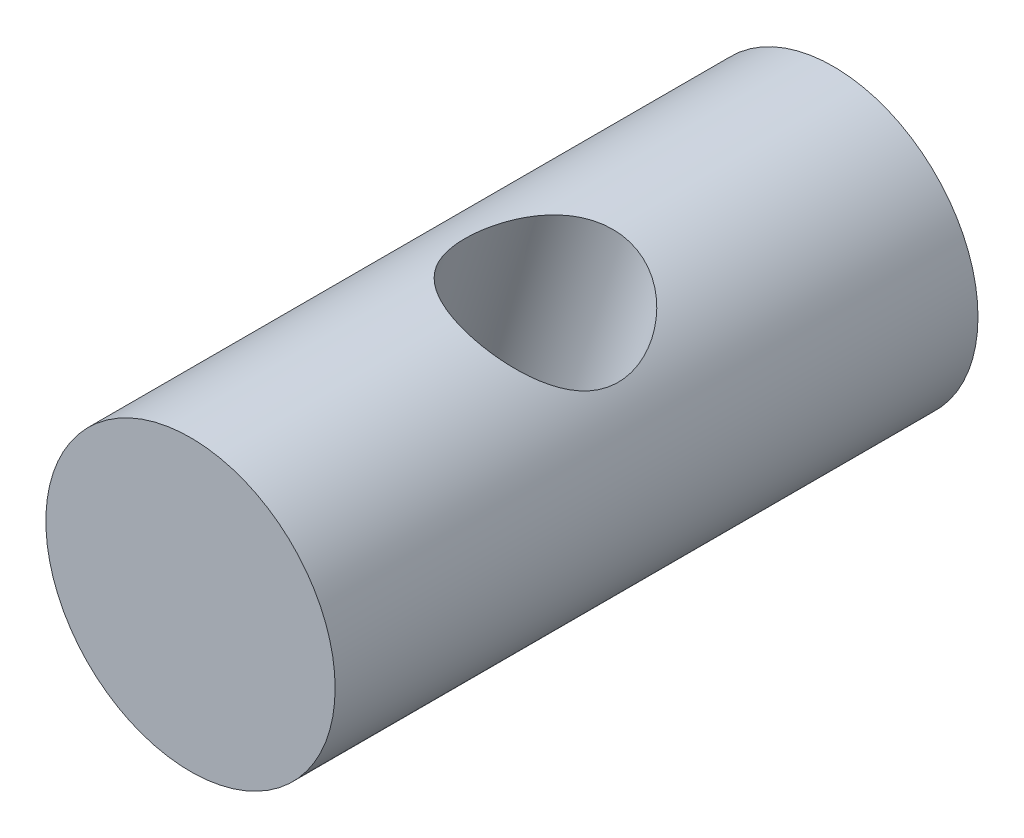
SolidWorks part; units mm, degrees
ref_plane "前视基准面" through (0, 0, 0) normal (0, 0, 1) x (1, 0, 0)
ref_plane "上视基准面" through (0, 0, 0) normal (0, 1, 0) x (1, 0, 0)
ref_plane "右视基准面" through (0, 0, 0) normal (1, 0, 0) x (0, 0, -1)
sketch "草图1" plane through (0, 0, 0) normal (0, 0, 1) x (1, 0, 0)
  circle A0 centre (0, 0) radius 4.5
  dimension "D1" = 9
extrude "凸台-拉伸1" add sketch "草图1" along normal blind 20
ref_plane "基准面1" through (4.5, 0, 0) normal (1, 0, 0) x (0, -1, 0)
hole_wizard "M6 螺纹孔1" positions "3D草图1" profile "草图2" tap size "M6" standard "ISO"
sketch3d "3D草图1"
  point P0 (1.3351, 4.2974, 10.1897)
sketch "草图2" plane through (1.3351, 4.2974, 10.1897) normal (0, 0, 1) x (-0.955, 0.2967, 0)
  line L0 (0, 0) -> (0, 7.5022)
  line L1 (0, 7.5022) -> (2.5, 6)
  line L2 (2.5, 6) -> (2.5, 0)
  line L5 (2.5, 0) -> (0, 0)
  line L10 (0, 7.5022) -> (-2.5, 6) construction
  line L11 (0, -6.35) -> (0, 107.95) construction
  dimension "螺纹孔钻头直径" = 5
  dimension "螺纹孔钻头深度" = 6
  dimension "导头角度" = 118
cosmetic thread "孔螺蚊线1" parameters "D1"=12, "D2"=6
